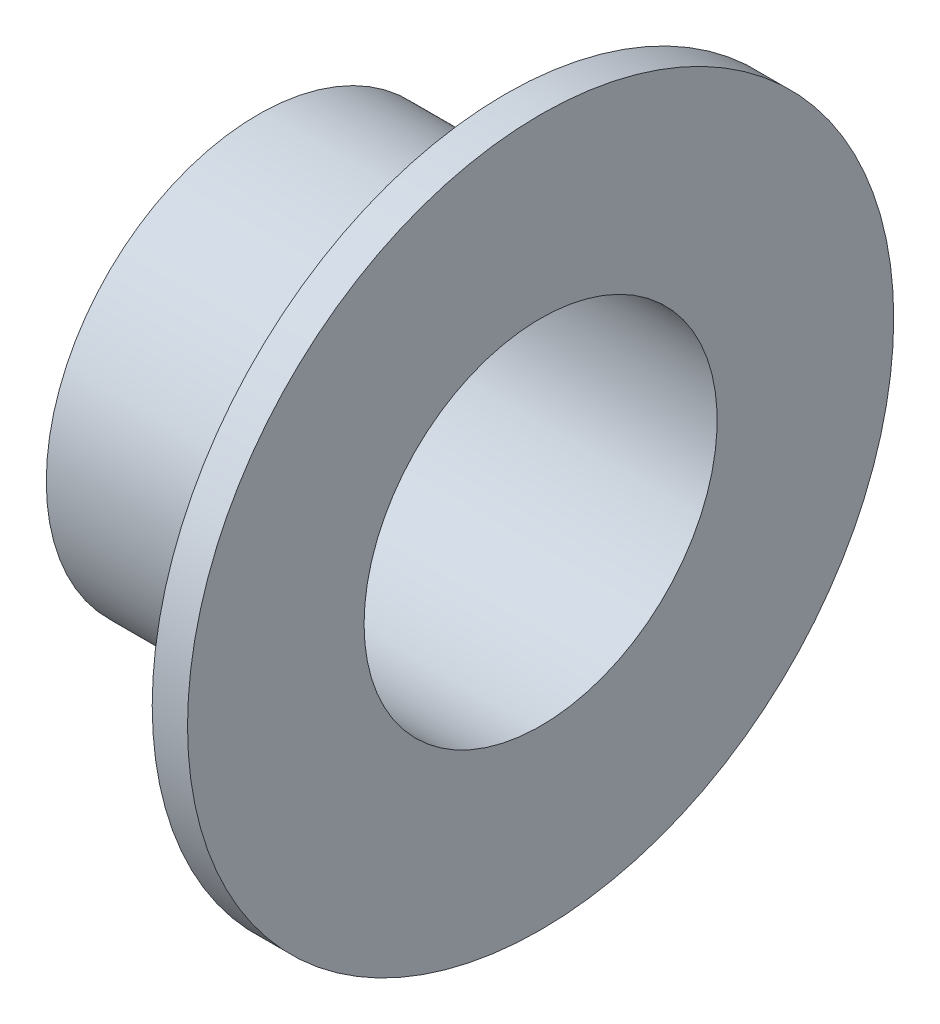
SolidWorks part; units mm, degrees
material "ABS"
ref_plane "前视基准面" through (0, 0, 0) normal (0, 0, 1) x (1, 0, 0)
ref_plane "上视基准面" through (0, 0, 0) normal (0, 1, 0) x (1, 0, 0)
ref_plane "右视基准面" through (0, 0, 0) normal (1, 0, 0) x (0, 0, -1)
other "Configuration Table"
sketch "草图1" plane through (0, 0, 0) normal (0, 1, 0) x (1, 0, 0)
  line L0 (-238.3632, 0) -> (11679.7956, 0) construction
  line L1 (0, 2.5) -> (0, 3)
  line L2 (0, 3) -> (3.5, 3)
  line L3 (3.5, 3) -> (3.5, 5)
  line L4 (3.5, 5) -> (4, 5)
  line L5 (4, 5) -> (4, 2.5)
  line L6 (4, 2.5) -> (0, 2.5)
  dimension "D1" = 4
  dimension "D2" = 0.5
  dimension "D3" = 5
  dimension "D4" = 6
  dimension "D5" = 10
revolve "旋转1" add sketch "草图1" angle 360 about L0
